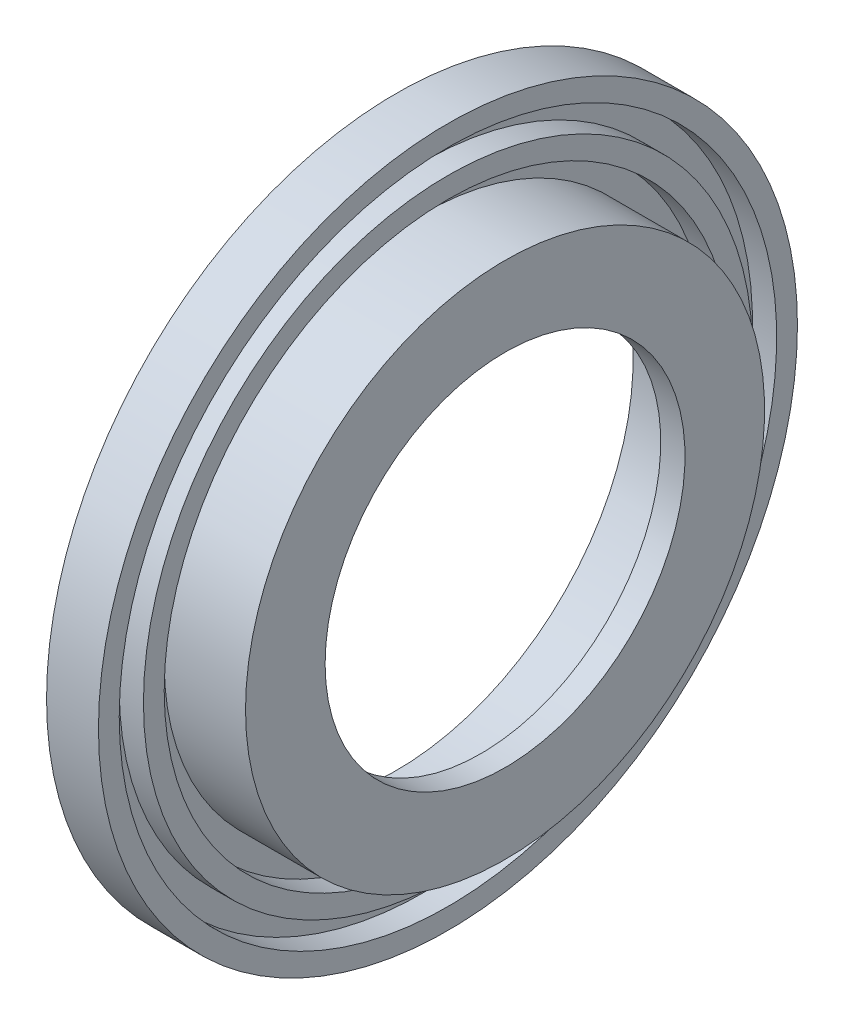
SolidWorks part; units mm, degrees
material "灰铸铁 HT150 "
ref_plane "Front Plane" through (0, 0, 0) normal (0, 0, 1) x (1, 0, 0)
ref_plane "Top Plane" through (0, 0, 0) normal (0, 1, 0) x (1, 0, 0)
ref_plane "Right Plane" through (0, 0, 0) normal (1, 0, 0) x (0, 0, -1)
sketch "Sketch2" plane through (0, 0, 0) normal (0, 0, 1) x (1, 0, 0)
  line L0 (0, 0) -> (171.2091, 0) construction
  line L1 (0, 137) -> (0, 202)
  line L2 (0, 202) -> (30, 202)
  line L3 (30, 202) -> (30, 190)
  line L4 (16, 150) -> (63, 150)
  line L5 (63, 150) -> (63, 104)
  line L6 (63, 104) -> (49, 104)
  line L7 (49, 104) -> (49, 137)
  line L8 (49, 137) -> (0, 137)
  line L13 (30, 176) -> (30, 164)
  line L14 (30, 190) -> (16, 190)
  line L15 (30, 176) -> (16, 176)
  line L16 (16, 190) -> (16, 176)
  line L18 (30, 164) -> (16, 164)
  line L20 (16, 164) -> (16, 150)
  dimension "D1" = 104
  dimension "D2" = 137
  dimension "D3" = 202
  dimension "D4" = 14
  dimension "D5" = 63
  dimension "D6" = 30
  dimension "D7" = 14
  dimension "D8" = 150
  dimension "D9" = 190
  dimension "D10" = 164
  dimension "D11" = 176
revolve "Revolve1" add sketch "Sketch2" angle 360 about L0
